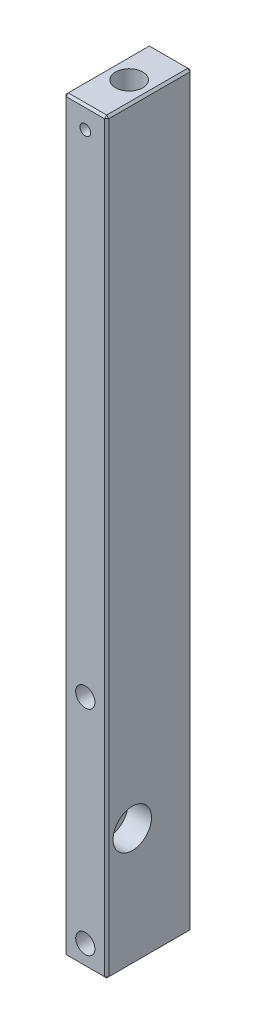
SolidWorks part; units mm, degrees
ref_plane "前视基准面" through (0, 0, 0) normal (0, 0, 1) x (1, 0, 0)
ref_plane "上视基准面" through (0, 0, 0) normal (0, 1, 0) x (1, 0, 0)
ref_plane "右视基准面" through (0, 0, 0) normal (1, 0, 0) x (0, 0, -1)
sketch "草图1" plane through (0, 0, 0) normal (0, 1, 0) x (1, 0, 0)
  line L1 (-10, -20) -> (10, -20)
  line L2 (-10, -20) -> (-10, 20)
  line L3 (-10, 20) -> (10, 20)
  line L4 (10, -20) -> (10, 20)
  line L5 (-10, -20) -> (10, 20) construction
  line L6 (-10, 20) -> (10, -20) construction
  point P0 (0, 0)
  dimension "D1" = 40
  dimension "D2" = 20
extrude "凸台-拉伸1" add sketch "草图1" along normal blind 350
sketch "草图2" plane through (0, 350, 0) normal (0, 1, 0) x (1, 0, 0)
  line L0 (-10, -20) -> (10, -20) construction
  circle A0 centre (0, 0.52) radius 6.4
  dimension "D1" = 12.8
  dimension "D2" = 20.52
extrude "切除-拉伸1" cut sketch "草图2" against normal blind 20
hole_wizard "M6 螺纹孔1" positions "草图3" profile "草图4" tap size "M6" standard "GB" end condition through all
sketch "草图3" plane through (0, 0, -20) normal (0, 0, -1) x (-1, 0, 0)
  line L0 (-10, 350) -> (10, 350) construction
  point P0 (0, 340)
  point P5 (0, 350)
  dimension "D1" = 10
cosmetic thread "孔螺蚊线1" parameters "D2"=6
sketch "草图4" plane through (0, 340, -20) normal (1, 0, 0) x (0, 1, 0)
  line L0 (0, 0) -> (0, 40)
  line L1 (0, 40) -> (2.5, 40)
  line L2 (2.5, 40) -> (2.5, 0)
  line L5 (2.5, 0) -> (0, 0)
  line L11 (0, -6.35) -> (0, 107.95) construction
  dimension "通孔螺纹孔钻头直径" = 5
  dimension "通孔螺纹孔钻头深度" = 40
chamfer "倒角1" distance 1 angle 45 12 edges at (10, 175, -20) (-10, 175, -20) (-10, 175, 20) (0, 350, 20) (-10, 350, 0) (0, 350, -20) (10, 350, 0) (10, 175, 20) (0, 0, 20) (-10, 0, 0) (0, 0, -20) (10, 0, 0)
hole_wizard "打孔尺寸(%根据)内六角圆柱头螺钉的类型1" positions "草图7" profile "草图6" counterbore size "M8" standard "GB" end condition through all
sketch "草图7" plane through (0, 0, -20) normal (0, 0, -1) x (-1, 0, 0)
  line L0 (9, 0) -> (-9, 0) construction
  point P0 (0, 10)
  point P2 (0, 110)
  dimension "D1" = 10
  dimension "D2" = 100
sketch "草图6" plane through (0, 10, -20) normal (1, 0, 0) x (0, 1, 0)
  line L0 (0, 0) -> (0, 40)
  line L1 (0, 40) -> (4.5, 40)
  line L3 (4.5, 40) -> (4.5, 9)
  line L4 (4.5, 9) -> (7.5, 9)
  line L5 (7.5, 9) -> (7.5, 0)
  line L7 (7.5, 0) -> (0, 0)
  line L11 (0, -6.35) -> (0, 107.95) construction
  dimension "通孔孔直径" = 9
  dimension "通孔孔深度" = 40
  dimension "柱形沉头孔直径" = 15
  dimension "柱形沉头孔深度" = 9
hole_wizard "打孔尺寸(%根据)内六角圆柱头螺钉的类型2" positions "草图10" profile "草图11" counterbore size "M10" standard "GB"
sketch "草图10" plane through (10, 0, 0) normal (1, 0, 0) x (0, 0, -1)
  line L0 (-20, 1) -> (-20, 349) construction
  line L1 (-8, 111.3242) -> (-8, 55.6621) construction
  line L2 (-8, 55.6621) -> (-8, 0) construction
  line L3 (19, 0) -> (-19, 0) construction
  point P0 (-8, 55.6621)
  dimension "D1" = 12
sketch "草图11" plane through (10, 55.6621, 8) normal (0, 1, 0) x (0, 0, -1)
  line L0 (0, 0) -> (0, 53.3047)
  line L1 (0, 53.3047) -> (5.5, 50)
  line L2 (5.5, 50) -> (5.5, 11)
  line L3 (5.5, 11) -> (9, 11)
  line L4 (9, 11) -> (9, 0)
  line L5 (9, 0) -> (0, 0)
  line L10 (0, 53.3047) -> (-5.5, 50) construction
  line L11 (0, -6.35) -> (0, 107.95) construction
  dimension "孔直径" = 11
  dimension "孔深度" = 50
  dimension "柱形沉头孔直径" = 18
  dimension "柱形沉头孔深度" = 11
  dimension "导头角度" = 118
